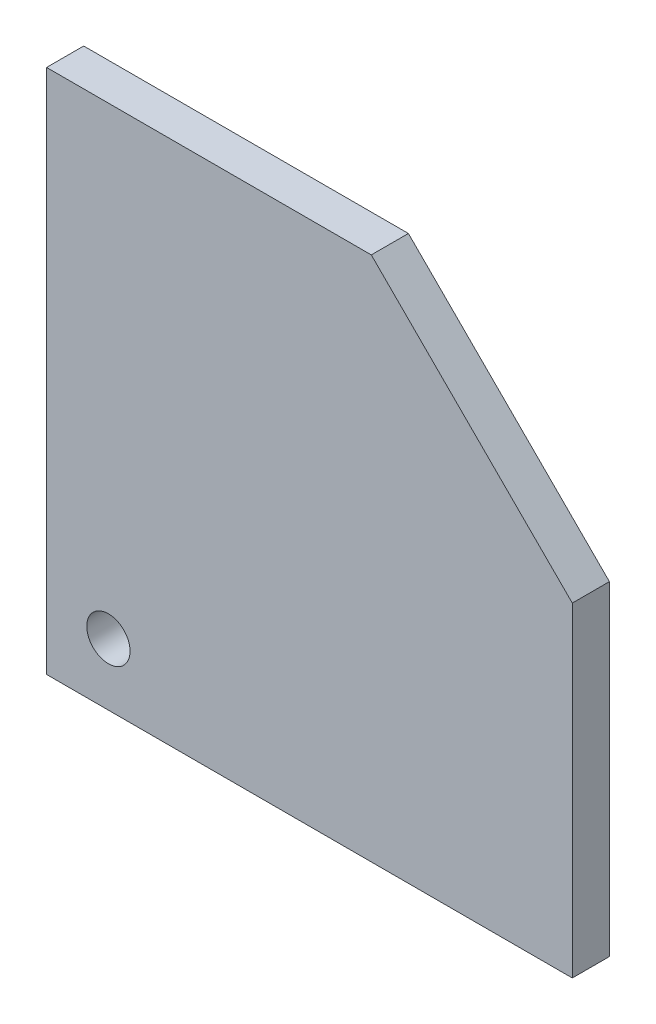
SolidWorks part; units mm, degrees
ref_plane "Front Plane" through (0, 0, 0) normal (0, 0, 1) x (1, 0, 0)
ref_plane "Top Plane" through (0, 0, 0) normal (0, 1, 0) x (1, 0, 0)
ref_plane "Right Plane" through (0, 0, 0) normal (1, 0, 0) x (0, 0, -1)
sketch "Sketch1" plane through (0, 0, 0) normal (0, 0, 1) x (1, 0, 0)
  line L1 (0, 0) -> (170, 0)
  line L2 (0, 0) -> (0, 170)
  line L3 (0, 170) -> (170, 170)
  line L4 (170, 0) -> (170, 170)
  point P6 (0, 0)
  dimension "D1" = 170
  dimension "D2" = 170
extrude "Extrude1" add sketch "Sketch1" against normal blind 12
hole_wizard "M16x2.0 Tapped Hole1" positions "Sketch3" profile "Sketch2" tap size "M16x2.0" standard "ISO" end condition through all
sketch "Sketch3" plane through (0, 0, 0) normal (0, 0, 1) x (1, 0, 0)
  line L1 (20, 170) -> (20, 0) construction
  line L2 (170, 170) -> (0, 170) construction
  line L3 (0, 0) -> (170, 0) construction
  line L4 (0, 20) -> (170, 20) construction
  line L5 (0, 170) -> (0, 0) construction
  line L6 (170, 0) -> (170, 170) construction
  point P12 (20, 20)
  dimension "D1" = 20
  dimension "D2" = 20
sketch "Sketch2" plane through (20, 20, 0) normal (1, 0, 0) x (0, -1, 0)
  line L0 (0, 0) -> (0, 12)
  line L1 (0, 12) -> (7, 12)
  line L2 (7, 12) -> (7, 0)
  line L5 (7, 0) -> (0, 0)
  line L11 (0, -6.35) -> (0, 107.95) construction
  dimension "貫穿螺孔鑽直徑" = 14
  dimension "貫穿螺孔鑽深度" = 12
cosmetic thread "Cosmetic Thread1" parameters "D1"=10, "D2"=16
hole_wizard "M8x1.25 Tapped Hole1" positions "Sketch7" profile "Sketch6" tap size "M8x1.25" standard "ISO"
sketch "Sketch7" plane through (0, 0, 0) normal (0, 0, 1) x (1, 0, 0)
  line L0 (170, 170) -> (0, 0) construction
  line L1 (109.7145, 189.5119) -> (197.5987, 101.6277) construction
  line L2 (62.6633, 151.7102) -> (173.1111, 41.2625) construction
  line L3 (183.6044, 127.0359) -> (116.4935, 59.925) construction
  line L4 (124.4377, 181.0062) -> (61.9619, 118.5304) construction
  line L5 (86.7476, 170.0524) -> (128.4, 128.4) construction
  line L6 (0, 170) -> (0, 0) construction
  line L7 (0, 0) -> (170, 0) construction
  point P16 (121.3289, 177.8975)
  point P17 (78.9025, 135.4711)
  point P18 (177.8975, 121.3289)
  point P19 (135.4711, 78.9025)
  dimension "D1" = 30
  dimension "D2" = 30
  dimension "D3" = 40
  dimension "D4" = 40
  dimension "D5" = 128.4
  dimension "D6" = 128.4
sketch "Sketch6" plane through (121.3289, 177.8975, 0) normal (1, 0, 0) x (0, -1, 0)
  line L0 (0, 0) -> (0, 12)
  line L1 (0, 12) -> (3.4, 12)
  line L2 (3.4, 12) -> (3.4, 0)
  line L5 (3.4, 0) -> (0, 0)
  line L11 (0, -6.35) -> (0, 107.95) construction
  dimension "貫穿螺孔鑽直徑" = 6.8
  dimension "貫穿螺孔鑽深度" = 12
cosmetic thread "Cosmetic Thread2" [suppressed] parameters "D1"=10, "D2"=8
cosmetic thread "Cosmetic Thread3" [suppressed] parameters "D1"=10, "D2"=8
cosmetic thread "Cosmetic Thread4" [suppressed] parameters "D1"=10, "D2"=8
cosmetic thread "Cosmetic Thread5" [suppressed] parameters "D1"=10, "D2"=8
chamfer "Chamfer1" distance 65 angle 45 1 edges at (170, 170, -6)
